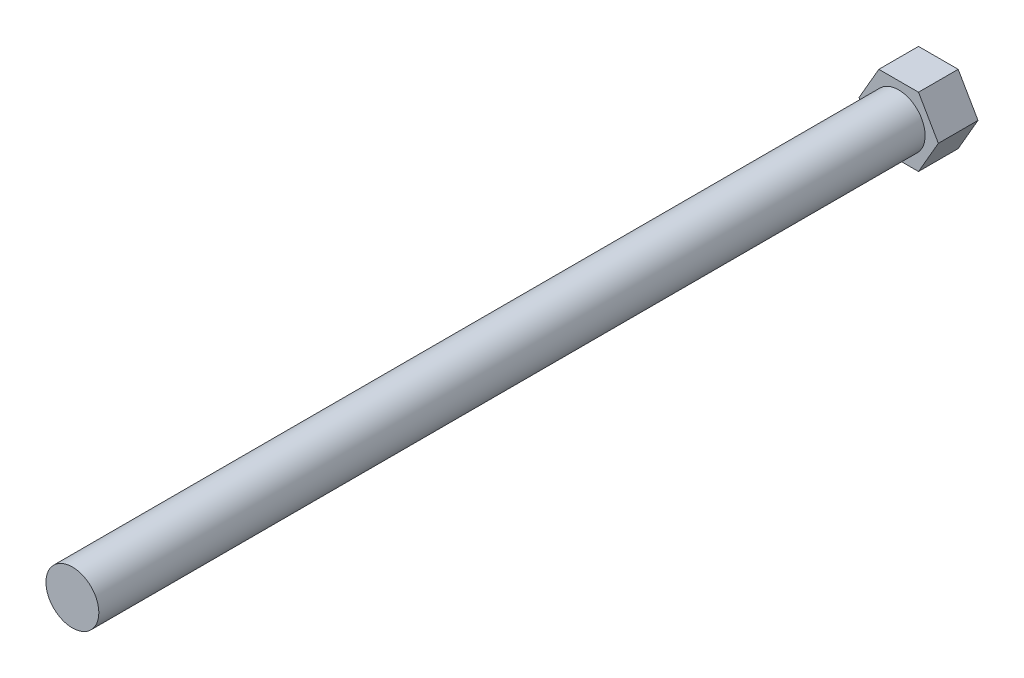
from build123d import *

# Parameters (mm, degrees)
SKETCH_1_R      = 8
EXTRUDE_1_DEPTH = 250
EXTRUDE_2_DEPTH = 12


with BuildPart() as part:
    # 草图1 → 凸台-拉伸1 (new body)
    with BuildSketch(Plane.XY):
        Circle(SKETCH_1_R)
    extrude(amount=EXTRUDE_1_DEPTH)

    # 草图2 → 凸台-拉伸2 (add)
    with BuildSketch(Plane.XY):
        Polygon((12, 0), (6, 10.392304845), (-6, 10.392304845), (-12, 0), (-6, -10.392304845), (6, -10.392304845), align=None)
    extrude(amount=-EXTRUDE_2_DEPTH)


solid = part.part
